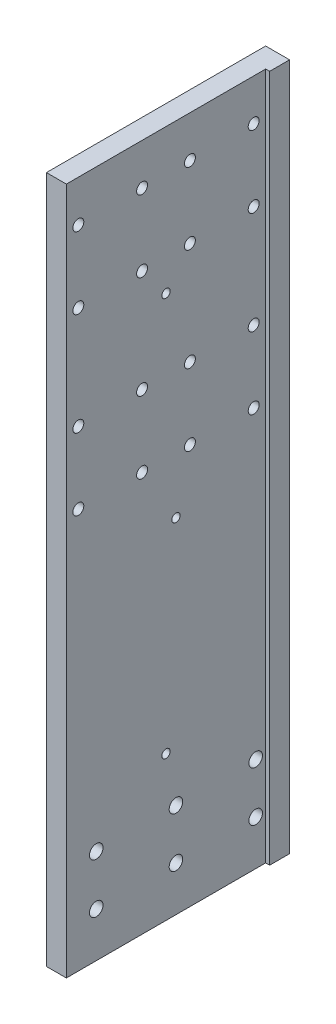
SolidWorks part; units mm, degrees
material "Q235A"
ref_plane "前视基准面" through (0, 0, 0) normal (0, 0, 1) x (1, 0, 0)
ref_plane "上视基准面" through (0, 0, 0) normal (0, 1, 0) x (1, 0, 0)
ref_plane "右视基准面" through (0, 0, 0) normal (1, 0, 0) x (0, 0, -1)
sketch "草图1" plane through (0, 0, 0) normal (1, 0, 0) x (0, 0, -1)
  line L1 (-55, -172.5) -> (55, -172.5)
  line L2 (-55, -172.5) -> (-55, 172.5)
  line L3 (-55, 172.5) -> (55, 172.5)
  line L4 (55, -172.5) -> (55, 172.5)
  line L5 (-55, -172.5) -> (55, 172.5) construction
  line L6 (-55, 172.5) -> (55, -172.5) construction
  point P0 (0, 0)
  dimension "D1" = 110
  dimension "D2" = 345
extrude "凸台-拉伸1" add sketch "草图1" along normal mid plane 12
sketch "草图2" plane through (6, 0, 0) normal (1, 0, 0) x (0, 0, -1)
  line L0 (-55, -172.5) -> (55, -172.5) construction
  line L1 (45, 172.5) -> (-55, 172.5)
  line L2 (45, 172.5) -> (45, -172.5)
  line L3 (45, -172.5) -> (-55, -172.5)
  line L4 (-55, 172.5) -> (-55, -172.5)
  line L5 (55, -172.5) -> (55, 172.5) construction
  line L6 (-55, 172.5) -> (-55, -172.5) construction
  line L7 (55, 172.5) -> (-55, 172.5) construction
  dimension "D1" = 10
extrude "切除-拉伸1" cut sketch "草图2" against normal blind 2
hole_wizard "M5 六角凹头螺钉的柱形沉头孔1" positions "草图3" profile "草图4" counterbore size "M5" standard "ISO" end condition through all
sketch "草图3" plane through (-6, 0, 0) normal (-1, 0, 0) x (0, 0, 1)
  line L6 (-55, 172.5) -> (55, 172.5) construction
  line L7 (-55, -172.5) -> (-55, 172.5) construction
  point P0 (-39, 151.75)
  point P3 (-7, 151.75)
  point P6 (17, 151.75)
  point P9 (49, 151.75)
  point P12 (49, 115.75)
  point P15 (17, 115.75)
  point P18 (-7, 115.75)
  point P21 (-39, 115.75)
  point P24 (-39, 64.25)
  point P27 (-7, 64.25)
  point P30 (17, 64.25)
  point P33 (49, 64.25)
  point P36 (-39, 28.25)
  point P39 (-7, 28.25)
  point P42 (17, 28.25)
  point P45 (49, 28.25)
  dimension "D1" = 32
  dimension "D2" = 56
  dimension "D3" = 88
  dimension "D4" = 36
  dimension "D5" = 87.5
  dimension "D6" = 123.5
  dimension "D7" = 20.75
  dimension "D8" = 16
sketch "草图4" plane through (-6, 151.75, -39) normal (0, 1, 0) x (0, 0, 1)
  line L0 (0, 0) -> (0, 12)
  line L1 (0, 12) -> (2.75, 12)
  line L3 (2.75, 12) -> (2.75, 5.4)
  line L4 (2.75, 5.4) -> (5, 5.4)
  line L5 (5, 5.4) -> (5, 0)
  line L7 (5, 0) -> (0, 0)
  line L11 (0, -6.35) -> (0, 107.95) construction
  dimension "通孔孔直径" = 5.5
  dimension "通孔孔深度" = 12
  dimension "柱形沉头孔直径" = 10
  dimension "柱形沉头孔深度" = 5.4
hole_wizard "M8 螺纹孔1" positions "草图5" profile "草图6" tap size "M8" standard "ISO" end condition through all
sketch "草图5" plane through (-6, 0, 0) normal (-1, 0, 0) x (0, 0, 1)
  line L0 (55, -172.5) -> (-55, -172.5) construction
  point P0 (-40, -125)
  point P3 (-40, -150)
  point P6 (0, -125)
  point P9 (0, -150)
  point P12 (40, -125)
  point P15 (40, -150)
  dimension "D1" = 40
  dimension "D2" = 40
  dimension "D3" = 25
  dimension "D4" = 47.5
sketch "草图6" plane through (-6, -125, -40) normal (0, 1, 0) x (0, 0, 1)
  line L0 (0, 0) -> (0, 12)
  line L1 (0, 12) -> (3.4, 12)
  line L2 (3.4, 12) -> (3.4, 0)
  line L5 (3.4, 0) -> (0, 0)
  line L11 (0, -6.35) -> (0, 107.95) construction
  dimension "通孔螺纹孔钻头直径" = 6.8
  dimension "通孔螺纹孔钻头深度" = 12
cosmetic thread "孔螺蚊线1" parameters "D2"=8
cosmetic thread "孔螺蚊线2" parameters "D2"=8
cosmetic thread "孔螺蚊线3" parameters "D2"=8
cosmetic thread "孔螺蚊线4" parameters "D2"=8
cosmetic thread "孔螺蚊线5" parameters "D2"=8
cosmetic thread "孔螺蚊线6" parameters "D2"=8
hole_wizard "M5 螺纹孔1" positions "草图7" profile "草图8" tap size "M5" standard "ISO" end condition through all
sketch "草图7" plane through (-6, 0, 0) normal (-1, 0, 0) x (0, 0, 1)
  line L1 (0, 0) -> (-107.8774, 0) construction
  line L2 (55, 172.5) -> (55, -172.5) construction
  point P0 (0, 0)
  point P10 (5, 100)
  point P12 (5, 185)
  point P22 (5, -100)
  dimension "D1" = 100
  dimension "D2" = 85
  dimension "D3" = 50
sketch "草图8" plane through (-6, 0, 0) normal (0, 1, 0) x (0, 0, 1)
  line L0 (0, 0) -> (0, 12)
  line L1 (0, 12) -> (2.1, 12)
  line L2 (2.1, 12) -> (2.1, 0)
  line L5 (2.1, 0) -> (0, 0)
  line L11 (0, -6.35) -> (0, 107.95) construction
  dimension "通孔螺纹孔钻头直径" = 4.2
  dimension "通孔螺纹孔钻头深度" = 12
cosmetic thread "孔螺蚊线7" parameters "D2"=5
cosmetic thread "孔螺蚊线10" parameters "D2"=5
cosmetic thread "孔螺蚊线11" parameters "D2"=5
hole_wizard "M6 螺纹孔1" positions "草图9" profile "草图10" tap size "M6" standard "ISO"
sketch "草图9" plane through (0, 0, -55) normal (0, 0, -1) x (-1, 0, 0)
  line L2 (-6, 172.5) -> (6, 172.5) construction
  point P4 (0, 157.5)
  point P7 (0, 120)
  point P10 (0, 82.5)
  point P13 (0, 45)
  point P16 (0, 7.5)
  dimension "D1" = 37.5
  dimension "D2" = 75
  dimension "D3" = 112.5
  dimension "D4" = 150
  dimension "D5" = 15
sketch "草图10" plane through (0, 157.5, -55) normal (1, 0, 0) x (0, 1, 0)
  line L0 (0, 0) -> (0, 16.5022)
  line L1 (0, 16.5022) -> (2.5, 15)
  line L2 (2.5, 15) -> (2.5, 0)
  line L5 (2.5, 0) -> (0, 0)
  line L10 (0, 16.5022) -> (-2.5, 15) construction
  line L11 (0, -6.35) -> (0, 107.95) construction
  dimension "螺纹孔钻头直径" = 5
  dimension "螺纹孔钻头深度" = 15
  dimension "导头角度" = 118
cosmetic thread "孔螺蚊线12" parameters "D1"=12, "D2"=6
cosmetic thread "孔螺蚊线13" parameters "D1"=12, "D2"=6
cosmetic thread "孔螺蚊线14" parameters "D1"=12, "D2"=6
cosmetic thread "孔螺蚊线15" parameters "D1"=12, "D2"=6
cosmetic thread "孔螺蚊线16" parameters "D1"=12, "D2"=6
